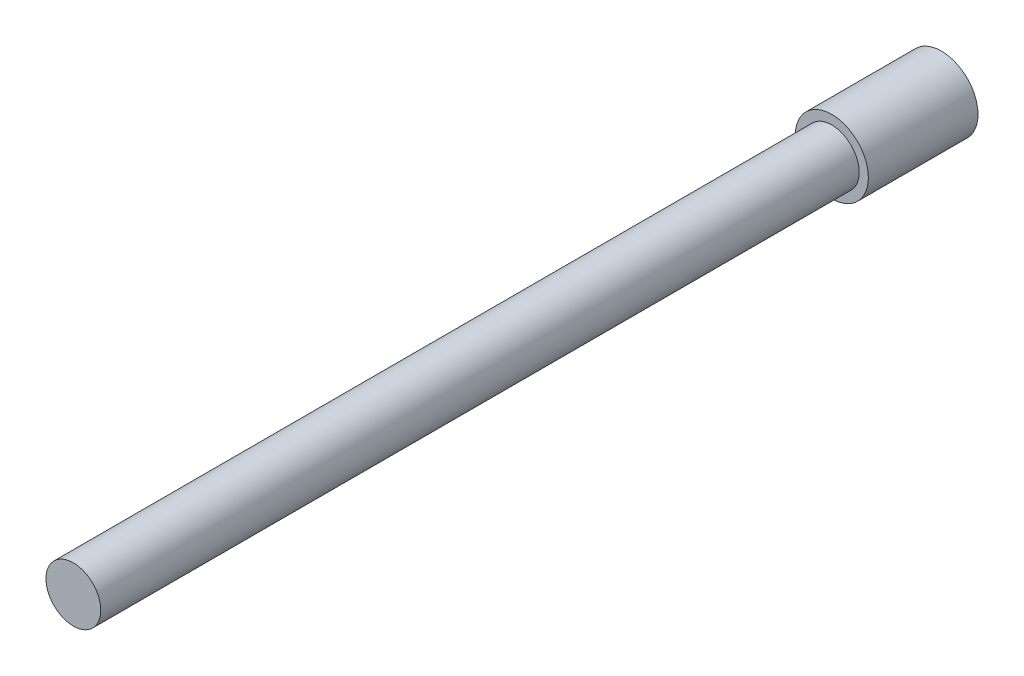
from build123d import *

# Parameters (mm, degrees)
SKETCH_1_R          = 4
EXTRUDE_1_DEPTH     = 95
CUT_EXTRUDE_START   = -83
SKETCH_2_R          = 4
SKETCH_2_R_2        = 3
CUT_EXTRUDE_1_DEPTH = 83


with BuildPart() as part:
    # 草图1 → 凸台-拉伸1 (new body)
    with BuildSketch(Plane.XY):
        Circle(SKETCH_1_R)
    extrude(amount=EXTRUDE_1_DEPTH)

    # 草图2 → 切除-拉伸1 (cut)
    with BuildSketch(Plane.XY.offset(95).offset(CUT_EXTRUDE_START)):
        Circle(SKETCH_2_R)
        Circle(SKETCH_2_R_2, mode=Mode.SUBTRACT)
    extrude(amount=CUT_EXTRUDE_1_DEPTH, mode=Mode.SUBTRACT)


solid = part.part
